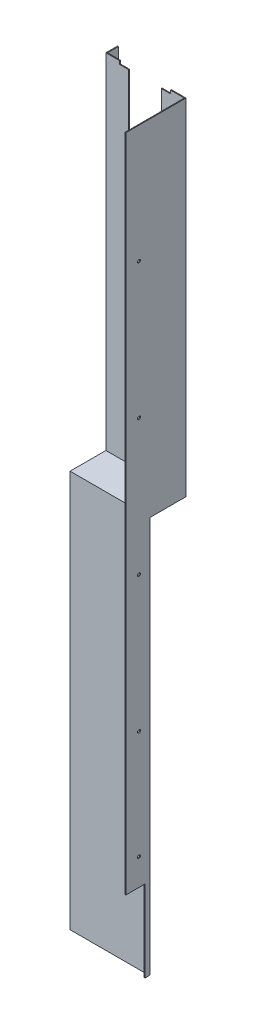
from build123d import *

# Parameters (mm, degrees)
SKETCH_1_W              = 146
SKETCH_1_H              = 636
EXTRUDE_1_DEPTH         = 1.5
SKETCH_3_W              = 1.5
SKETCH_3_H              = 636
EXTRUDE_3_DEPTH         = 109
SKETCH_4_W              = 144.5
SKETCH_4_H              = 1.5
EXTRUDE_4_DEPTH         = 66
EXTRUDE_5_DEPTH         = 730
SKETCH_6_W              = 1.5
SKETCH_6_H              = 634.5
EXTRUDE_6_DEPTH         = 20
SKETCH_7_W              = 1.5
SKETCH_7_H              = 730
EXTRUDE_7_DEPTH         = 10
SKETCH_8_W              = 1.5
SKETCH_8_H              = 56
EXTRUDE_8_DEPTH         = 10
SKETCH_9_W              = 35
SKETCH_9_H              = 150
CUT_EXTRUDE_1_DEPTH     = 2
CUT_EXTRUDE_2_DEPTH     = 2
HOLE_WIZARD_5_5_5_5_1_D = 5.5
HOLE_WIZARD_5_5_5_5_2_D = 5.5


with BuildPart() as part:
    # 草图1 → 凸台-拉伸1 (new body)
    with BuildSketch(Plane.XY):
        with Locations((73, 318)):
            Rectangle(SKETCH_1_W, SKETCH_1_H)
    extrude(amount=EXTRUDE_1_DEPTH)

    # 草图3 → 凸台-拉伸3 (add)
    with BuildSketch(Plane.XY.offset(1.5)):
        with Locations((145.25, 318)):
            Rectangle(SKETCH_3_W, SKETCH_3_H)
    extrude(amount=EXTRUDE_3_DEPTH)

    # 草图4 → 凸台-拉伸4 (add)
    with BuildSketch(Plane.XY.offset(1.5)):
        with Locations((72.25, 0.75)):
            Rectangle(SKETCH_4_W, SKETCH_4_H)
    extrude(amount=EXTRUDE_4_DEPTH)

    # 草图5 → 凸台-拉伸5 (add)
    with BuildSketch(Plane.XZ):
        Polygon((0, 67.5), (144.5, 67.5), (144.5, 110.5), (146, 110.5), (146, 66), (0, 66), align=None)
    extrude(amount=EXTRUDE_5_DEPTH)

    # 草图6 → 凸台-拉伸6 (add)
    with BuildSketch(Plane(origin=(0, 0, 0), x_dir=(-1, 0, 0), z_dir=(0, 0, -1))):
        with Locations((-0.75, 318.75)):
            Rectangle(SKETCH_6_W, SKETCH_6_H)
    extrude(amount=EXTRUDE_6_DEPTH)

    # 草图7 → 凸台-拉伸7 (add)
    with BuildSketch(Plane(origin=(0, 0, 66), x_dir=(-1, 0, 0), z_dir=(0, 0, -1))):
        with Locations((-0.75, -365)):
            Rectangle(SKETCH_7_W, SKETCH_7_H)
    extrude(amount=EXTRUDE_7_DEPTH)

    # 草图8 → 凸台-拉伸8 (add)
    with BuildSketch(Plane.XZ):
        with Locations((0.75, 28)):
            Rectangle(SKETCH_8_W, SKETCH_8_H)
    extrude(amount=EXTRUDE_8_DEPTH)

    # 草图9 → 切除-拉伸1 (cut)
    with BuildSketch(Plane.ZY.offset(-144.5)):
        with Locations((93, -655)):
            Rectangle(SKETCH_9_W, SKETCH_9_H)
    extrude(amount=-CUT_EXTRUDE_1_DEPTH, mode=Mode.SUBTRACT)

    # 草图10 → 切除-拉伸2 (cut)
    with BuildSketch(Plane.XY.offset(1.5)):
        Polygon((25, 636), (119, 636), (119, 630), (102, 630), (102, 501), (42, 501), (42, 630), (25, 630), align=None)
    extrude(amount=-CUT_EXTRUDE_2_DEPTH, mode=Mode.SUBTRACT)

    # Ø5.5 (5.5) 直径孔1 (through all)
    with Locations(Plane.ZY.offset(-144.5)):
        with Locations((86.5, 419), (86.5, 169), (86.5, -81), (86.5, -331), (86.5, -531)):
            Hole(HOLE_WIZARD_5_5_5_5_1_D / 2)

    # Ø5.5 (5.5) 直径孔2 (through all)
    with Locations(Plane.ZY):
        with Locations((-10, 301.5), (-10, 101.5)):
            Hole(HOLE_WIZARD_5_5_5_5_2_D / 2)


solid = part.part
